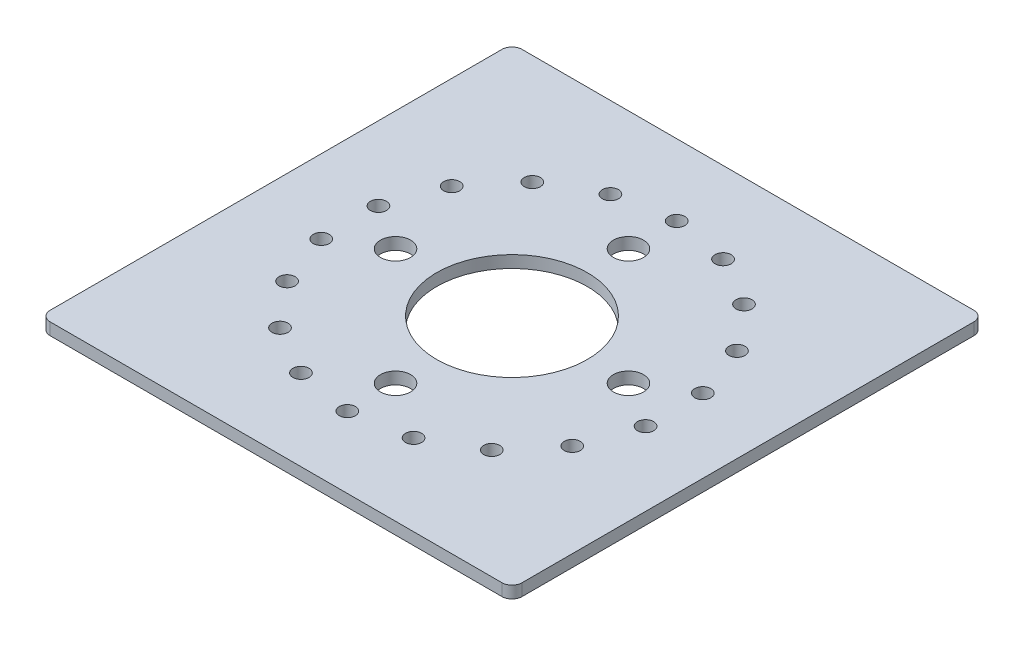
SolidWorks part; units mm, degrees
material "Q235B"
ref_plane "Front Plane" through (0, 0, 0) normal (0, 0, 1) x (1, 0, 0)
ref_plane "Top Plane" through (0, 0, 0) normal (0, 1, 0) x (1, 0, 0)
ref_plane "Right Plane" through (0, 0, 0) normal (1, 0, 0) x (0, 0, -1)
sketch "Sketch1" plane through (0, 0, 0) normal (0, 1, 0) x (1, 0, 0)
  line L1 (225, -235) -> (-225, -235)
  line L2 (235, -225) -> (235, 225)
  line L3 (225, 235) -> (-225, 235)
  line L4 (-235, -225) -> (-235, 225)
  line L5 (235, -235) -> (-235, 235) construction
  line L6 (235, 235) -> (-235, -235) construction
  arc A0 (-225, -235) -> (-235, -225) centre (-225, -225) cw
  arc A1 (235, 225) -> (225, 235) centre (225, 225) ccw
  arc A2 (225, -235) -> (235, -225) centre (225, -225) ccw
  arc A3 (-225, 235) -> (-235, 225) centre (-225, 225) ccw
  circle A4 centre (0, 0) radius 75
  point P0 (0, 0)
  dimension "D2" = 10
  dimension "D3" = 150
  dimension "D1" = 470
extrude "Boss-Extrude1" add sketch "Sketch1" along normal blind 12
hole_wizard "Ø16.0 (16) Diameter Hole1" positions "Sketch2" profile "Sketch3" hole size "Ø16.0" standard "GB" end condition up to next
sketch "Sketch2" plane through (0, 12, 0) normal (0, 1, 0) x (1, 0, 0)
  circle A0 centre (0, 0) radius 164 construction
  point P0 (0, 164)
  point P13 (56.0913, 154.1096)
  point P14 (105.4172, 125.6313)
  point P15 (142.0282, 82)
  point P16 (161.5085, 28.4783)
  point P17 (161.5085, -28.4783)
  point P18 (142.0282, -82)
  point P19 (105.4172, -125.6313)
  point P20 (56.0913, -154.1096)
  point P21 (0, -164)
  point P22 (-56.0913, -154.1096)
  point P23 (-105.4172, -125.6313)
  point P24 (-142.0282, -82)
  point P25 (-161.5085, -28.4783)
  point P26 (-161.5085, 28.4783)
  point P27 (-142.0282, 82)
  point P28 (-105.4172, 125.6313)
  point P29 (-56.0913, 154.1096)
  dimension "D1" = 328
  dimension "D2" = 18
sketch "Sketch3" plane through (0, 12, -164) normal (1, 0, 0) x (0, 0, 1)
  line L0 (0, 0) -> (0, 12)
  line L1 (0, 12) -> (8, 12)
  line L2 (8, 12) -> (8, 0)
  line L5 (8, 0) -> (0, 0)
  line L11 (0, -6.35) -> (0, 107.95) construction
  dimension "通孔孔直径" = 16
  dimension "通孔孔深度" = 12
hole_wizard "Ø30 Diameter Hole2" positions "Sketch4" profile "Sketch5" hole size "Ø16.0" standard "GB" end condition up to next
sketch "Sketch4" plane through (0, 12, 0) normal (0, 1, 0) x (1, 0, 0)
  circle A0 centre (0, 0) radius 116 construction
  point P0 (0, 116)
  point P11 (116, 0)
  point P12 (0, -116)
  point P13 (-116, 0)
  dimension "D1" = 232
  dimension "D2" = 4
sketch "Sketch5" plane through (0, 12, -116) normal (1, 0, 0) x (0, 0, 1)
  line L0 (0, 0) -> (0, 12)
  line L1 (0, 12) -> (15, 12)
  line L2 (15, 12) -> (15, 0)
  line L5 (15, 0) -> (0, 0)
  line L11 (0, -6.35) -> (0, 107.95) construction
  dimension "通孔孔直径" = 30
  dimension "通孔孔深度" = 12
